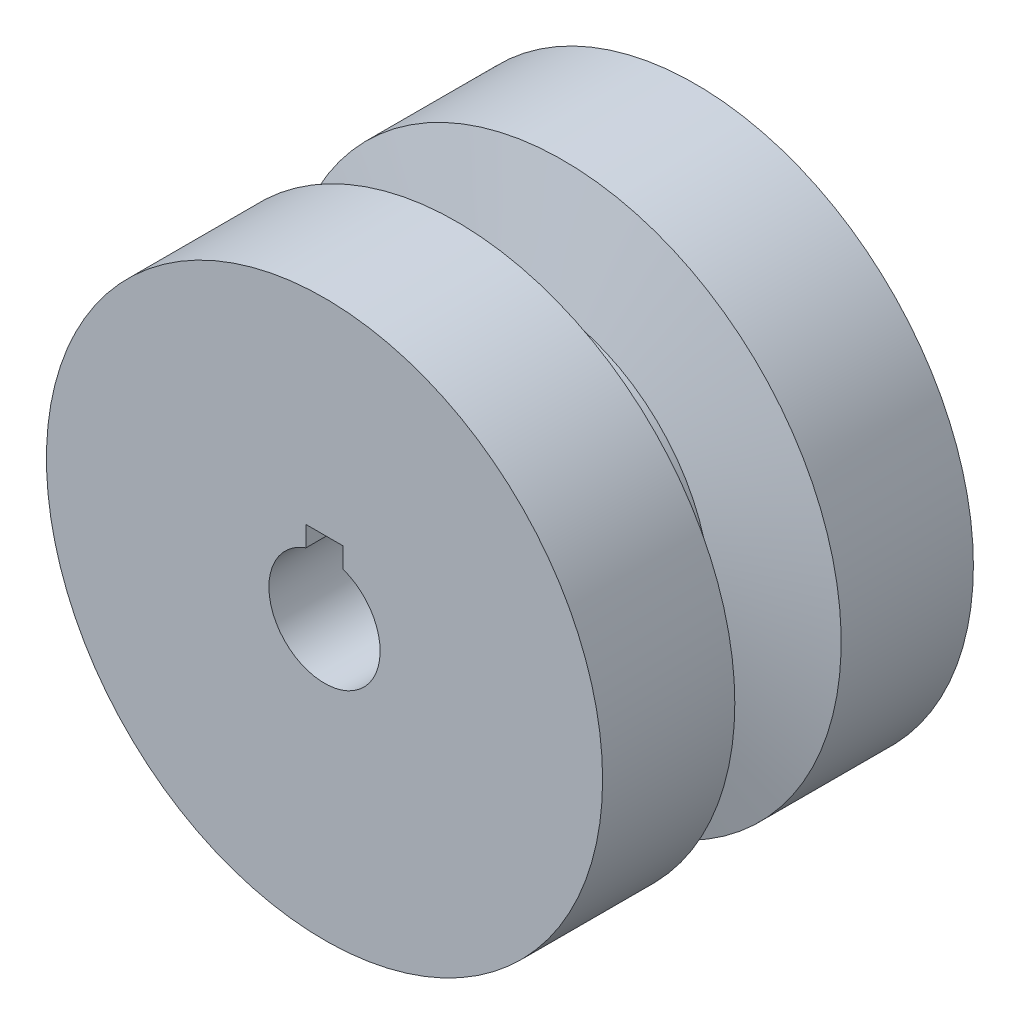
from build123d import *

# Parameters (mm, degrees)
SKETCH_1_R          = 37.5
SKETCH_1_R_2        = 7.5
EXTRUDE_1_DEPTH     = 50
SKETCH_7_W          = 5
SKETCH_7_H          = 4.6
CUT_EXTRUDE_1_DEPTH = 90


with BuildPart() as part:
    # 草图1 → 凸台-拉伸1 (new body)
    with BuildSketch(Plane.XY):
        Circle(SKETCH_1_R)
        Circle(SKETCH_1_R_2, mode=Mode.SUBTRACT)
    extrude(amount=EXTRUDE_1_DEPTH)

    # 草图2 → 切除-旋转1 (revolve, cut)
    with BuildSketch(Plane(origin=(0, 0, 0), x_dir=(1, 0, 0), z_dir=(0, 1, 0))):
        Polygon((-38.25, -17.648818614), (-23.25, -21.25), (-23.25, -28.75), (-38.25, -32.351181386), align=None)
    revolve(axis=Axis((0, 0, 0), (0, 0, 1)), mode=Mode.SUBTRACT)

    # 草图3 → M5 螺纹孔2 (revolve, cut)
    with BuildSketch(Plane(origin=(0, 32.5, 9), x_dir=(0, 0, 1), z_dir=(1, 0, 0))):
        Polygon((0, 0), (0, 31.2618073), (2.1, 30), (2.1, 0), align=None)
    revolve(axis=Axis((0, 38.85, 9), (0, -1, 0)), mode=Mode.SUBTRACT)

    # 草图5 → M5 螺纹孔1 (revolve, cut)
    with BuildSketch(Plane(origin=(32.5, 0, 9), x_dir=(0, 0, -1), z_dir=(0, 1, 0))):
        Polygon((0, 0), (0, 31.2618073), (2.1, 30), (2.1, 0), align=None)
    revolve(axis=Axis((38.85, 0, 9), (-1, 0, 0)), mode=Mode.SUBTRACT)

    # 草图7 → 切除-拉伸1 (cut)
    with BuildSketch(Plane(origin=(0, 0, 0), x_dir=(-1, 0, 0), z_dir=(0, 0, -1))):
        with Locations((0, 7.5)):
            Rectangle(SKETCH_7_W, SKETCH_7_H)
    extrude(amount=-CUT_EXTRUDE_1_DEPTH, mode=Mode.SUBTRACT)


solid = part.part
